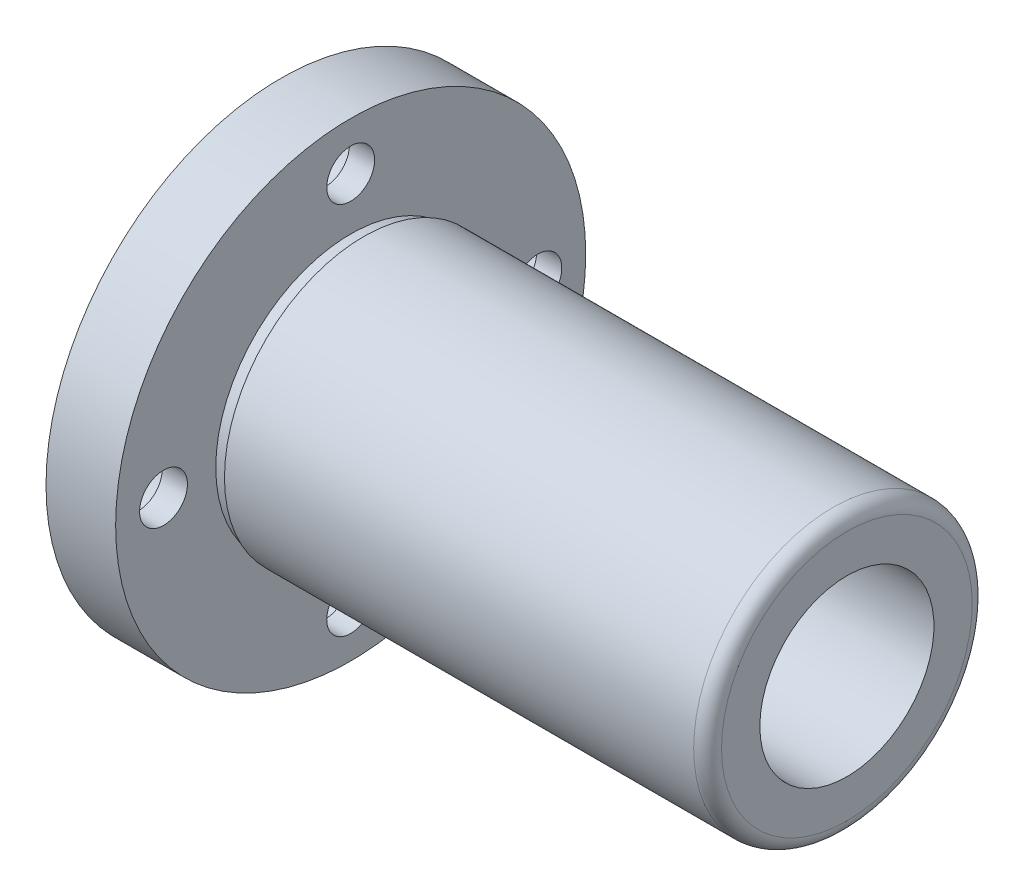
SolidWorks part; units mm, degrees
ref_plane "前视基准面" through (0, 0, 0) normal (0, 0, 1) x (1, 0, 0)
ref_plane "上视基准面" through (0, 0, 0) normal (0, 1, 0) x (1, 0, 0)
ref_plane "右视基准面" through (0, 0, 0) normal (1, 0, 0) x (0, 0, -1)
sketch "草图1" plane through (0, 0, 0) normal (0, 0, 1) x (1, 0, 0)
  line L0 (0, 27) -> (0, 10)
  line L1 (0, 10) -> (65, 10)
  line L2 (65, 10) -> (65, 14.4)
  line L3 (63.4, 16) -> (9.5, 16)
  line L4 (9.5, 16) -> (9.5, 15.5)
  line L5 (9.5, 15.5) -> (8, 15.5)
  line L6 (8, 15.5) -> (8, 27)
  line L7 (8, 27) -> (0, 27)
  line L8 (65, 0) -> (0, 0) construction
  arc A0 (65, 14.4) -> (63.4, 16) centre (63.4, 14.4) ccw
revolve "旋转1" add sketch "草图1" angle 360 about L8
sketch "草图2" plane through (0, 0, 0) normal (0, 0, 1) x (1, 0, 0)
  line L0 (0, 21.5) -> (0, 26)
  line L1 (0, 26) -> (5.1, 26)
  line L2 (5.1, 26) -> (5.1, 24.25)
  line L3 (5.1, 24.25) -> (8, 24.25)
  line L4 (8, 24.25) -> (8, 21.5)
  line L5 (8, 21.5) -> (0, 21.5)
  line L6 (8, 21.5) -> (0, 21.5) construction
revolve "切除-旋转1" cut sketch "草图2" angle 360 about L6
sketch "草图3" plane through (0, 0, 0) normal (1, 0, 0) x (0, 0, -1)
  line L0 (0, 21.5) -> (-707.1068, -685.6068)
  line L1 (0, 21.5) -> (707.1068, -685.6068)
pattern_linear "阵列(线性)1" count 2 spacing 30.4056 along (0, -0.7071, 0.7071) count 2 spacing 30.4056 along (0, -0.7071, -0.7071) of "切除-旋转1"
